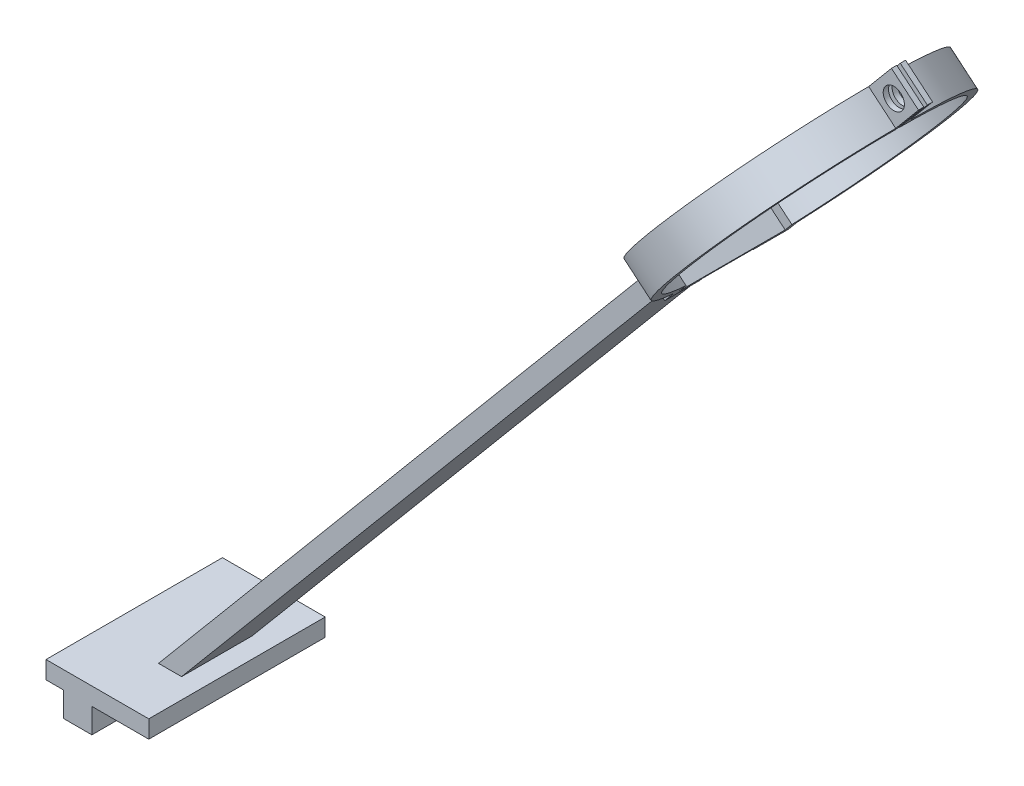
SolidWorks part; units mm, degrees
material "铜"
ref_plane "前视基准面" through (0, 0, 0) normal (0, 0, 1) x (1, 0, 0)
ref_plane "上视基准面" through (0, 0, 0) normal (0, 1, 0) x (1, 0, 0)
ref_plane "右视基准面" through (0, 0, 0) normal (1, 0, 0) x (0, 0, -1)
sketch "草图1" plane through (0, 0, 0) normal (0, 0, 1) x (1, 0, 0)
  line L1 (0, 0) -> (138.1993, 164.6996)
  line L3 (10.7225, 5) -> (142.0296, 161.4856)
  line L6 (138.1993, 164.6996) -> (145.27, 173.126)
  line L7 (145.27, 173.126) -> (149.1002, 169.9121)
  line L8 (149.1002, 169.9121) -> (142.0296, 161.4856)
  line L9 (0, 0) -> (-6.4279, -7.6604)
  line L10 (-6.4279, -7.6604) -> (30, -7.6604)
  line L11 (30, -2.6604) -> (30, -7.6604)
  line L12 (30, -2.6604) -> (4.2947, -2.6604)
  line L13 (4.2947, -2.6604) -> (10.7225, 5)
  line L15 (0, 0) -> (30, 0) construction
  line L16 (10.7225, 5) -> (30, 5) construction
  dimension "D1" = 5
  dimension "D2" = 215
  dimension "D5" = 11
  dimension "D6" = 10
  dimension "D4" = 5
extrude "凸台-拉伸1" add sketch "草图1" along normal mid plane 20
ref_plane "基准面1" through (0, 0, 0) normal (-0.766, 0.6428, 0) x (0, 0, 1)
sketch "草图2" plane through (0, 0, 0) normal (-0.766, 0.6428, 0) x (0, 0, 1)
sketch "草图3" plane through (0, 0, 0) normal (-0.766, 0.6428, 0) x (0, 0, 1)
  line L3 (0, 261.2432) -> (0, 226.2432) construction
  line L10 (15, 226.2432) -> (15, 227.9678)
  line L12 (0, 297.7432) -> (0, 261.2432) construction
  line L16 (-15, 227.9678) -> (-15, 226.2432)
  line L17 (-15, 226.2432) -> (-15, 225)
  line L18 (-15, 225) -> (-10, 225)
  line L19 (-10, 226) -> (-10, -10) construction
  line L20 (-10, 225) -> (-10, 226)
  line L21 (-10, 226) -> (10, 226)
  line L22 (10, 226) -> (10, 225)
  line L23 (10, 226) -> (10, -10) construction
  line L24 (10, 225) -> (15, 225)
  line L25 (15, 225) -> (15, 226.2432)
  arc A2 (15, 227.9678) -> (-15, 227.9678) centre (0, 261.2432) ccw
  point P9 (0, 211)
  dimension "D1" = 73
  dimension "D2" = 1
extrude "拉伸-薄壁2" add sketch "草图3" along normal blind 5 and the other way blind 5 from offset 2.5 thin offset against normal yes
sketch "草图4" plane through (0, 0, 0) normal (-0.766, 0.6428, 0) x (0, 0, 1)
  line L0 (10, 226) -> (10, 225) construction
  line L5 (-10, 225) -> (10, 225)
  line L6 (-10, 225) -> (-10, 227.7008)
  line L7 (-10, 227.7008) -> (10, 227.7008)
  line L8 (10, 225) -> (10, 227.7008)
extrude "切除-拉伸3" cut sketch "草图4" against normal through all both and the other way through all
sketch "草图5" plane through (0, 0, 0) normal (-0.766, 0.6428, 0) x (0, 0, 1)
  line L1 (-0.5, 290.2916) -> (0.5, 290.2916)
  line L2 (-0.5, 290.2916) -> (-0.5, 305.1948)
  line L3 (-0.5, 305.1948) -> (0.5, 305.1948)
  line L4 (0.5, 290.2916) -> (0.5, 305.1948)
  line L5 (-0.5, 290.2916) -> (0.5, 305.1948) construction
  line L6 (-0.5, 305.1948) -> (0.5, 290.2916) construction
  arc A0 (15, 227.9678) -> (-15, 227.9678) centre (0, 261.2432) ccw construction
  point P0 (0, 297.7432)
  dimension "D1" = 1
extrude "切除-拉伸2" cut sketch "草图5" against normal through all both and the other way through all
ref_plane "基准面2" through (192.9905, 229.9972, 0) normal (0.6428, 0.766, 0) x (0.766, -0.6428, 0)
sketch "草图8" plane through (192.9905, 229.9972, 0) normal (0.6428, 0.766, 0) x (0.766, -0.6428, 0)
  line L0 (-2.5, -0.5) -> (-2.5, -39) construction
  line L1 (7.5, -0.5) -> (-2.5, -0.5)
  line L2 (7.5, -0.5) -> (7.5, -2)
  line L3 (7.5, -2) -> (-2.5, -2)
  line L4 (-2.5, -0.5) -> (-2.5, -2)
  dimension "D1" = 1.5
extrude "凸台-拉伸2" add sketch "草图8" along normal blind 10 and the other way up to body
mirror "镜向1" about plane through (0, 0, 0) normal (0, 0, 1) of "凸台-拉伸2"
sketch "草图11" plane through (0, -7.6604, 0) normal (0, -1, 0) x (1, 0, 0)
  line L1 (30, 10) -> (10, 10)
  line L2 (30, 10) -> (30, -16.0035)
  line L3 (30, -16.0035) -> (10, -16.0035)
  line L4 (10, 10) -> (10, -16.0035)
  dimension "D1" = 20
extrude "切除-拉伸4" cut sketch "草图11" against normal blind 10
sketch "草图12" plane through (0, 0, 10) normal (0, 0, 1) x (1, 0, 0)
  line L0 (4.2947, -2.6604) -> (-2.2324, -2.6604)
  line L6 (10, -7.6604) -> (10, -2.6604)
  line L7 (10, -2.6604) -> (4.2947, -2.6604)
  line L8 (4.2947, -2.6604) -> (146.8505, 167.231)
  line L9 (146.8505, 167.231) -> (143.0202, 170.4449)
  line L10 (143.0202, 170.4449) -> (-6.4279, -7.6604)
  line L11 (-6.4279, -7.6604) -> (10, -7.6604)
  line L12 (10, -7.6604) -> (10, -2.6604)
  line L13 (10, -2.6604) -> (4.2947, -2.6604)
  line L15 (146.8505, 167.231) -> (143.0202, 170.4449)
  line L16 (-2.2324, -2.6604) -> (-6.4279, -7.6604)
  line L17 (-6.4279, -7.6604) -> (10, -7.6604)
  dimension "D1" = 0
extrude "凸台-拉伸3" add sketch "草图12" along normal blind 15 contours L12 L13 L0 L16 L17
mirror "镜向2" about plane through (0, 0, 0) normal (0, 0, 1) of "凸台-拉伸3"
sketch "草图13" plane through (0, 0, -2) normal (0, 0, -1) x (-1, 0, 0)
  line L0 (-201.3335, 236.0507) -> (-198.1638, 232.2076) construction
  line L1 (-197.5033, 239.2646) -> (-205.1638, 232.8367) construction
  line L2 (-194.2739, 235.4159) -> (-198.1638, 232.2076) construction
  line L3 (-191.0445, 231.5673) -> (-197.5033, 239.2646) construction
  circle A0 centre (-198.1638, 232.2076) radius 3
  dimension "D1" = 6
extrude "切除-拉伸5" cut sketch "草图13" against normal through all both and the other way through all
sketch "草图14" plane through (0, 0, -25) normal (0, 0, -1) x (-1, 0, 0)
  line L0 (2.2324, -2.6604) -> (6.4279, -2.6604)
  line L2 (6.4279, -2.6604) -> (14.1279, -2.6604)
  line L5 (14.1279, -14.6604) -> (6.4279, -14.6604)
  line L7 (6.4279, -7.6604) -> (2.2324, -2.6604)
  line L8 (6.1279, -7.6604) -> (6.1279, -14.6604)
  line L9 (6.4279, -7.6604) -> (-10, -7.6604) construction
  line L10 (6.1279, -14.6604) -> (6.4279, -14.6604)
  line L11 (6.4279, -7.6604) -> (6.1279, -7.6604)
  line L12 (14.1279, -7.6604) -> (14.1279, -14.6604)
  line L13 (14.1279, -7.6604) -> (19.1279, -7.6604)
  line L14 (19.1279, -7.6604) -> (19.1279, -2.6604)
  line L15 (19.1279, -2.6604) -> (14.1279, -2.6604)
  dimension "D1" = 8
  dimension "D2" = 5
  dimension "D3" = 0.3
extrude "凸台-拉伸4" add sketch "草图14" against normal up to surface (50 mm away) up to face at (2.8349, -5.1604, 25)
